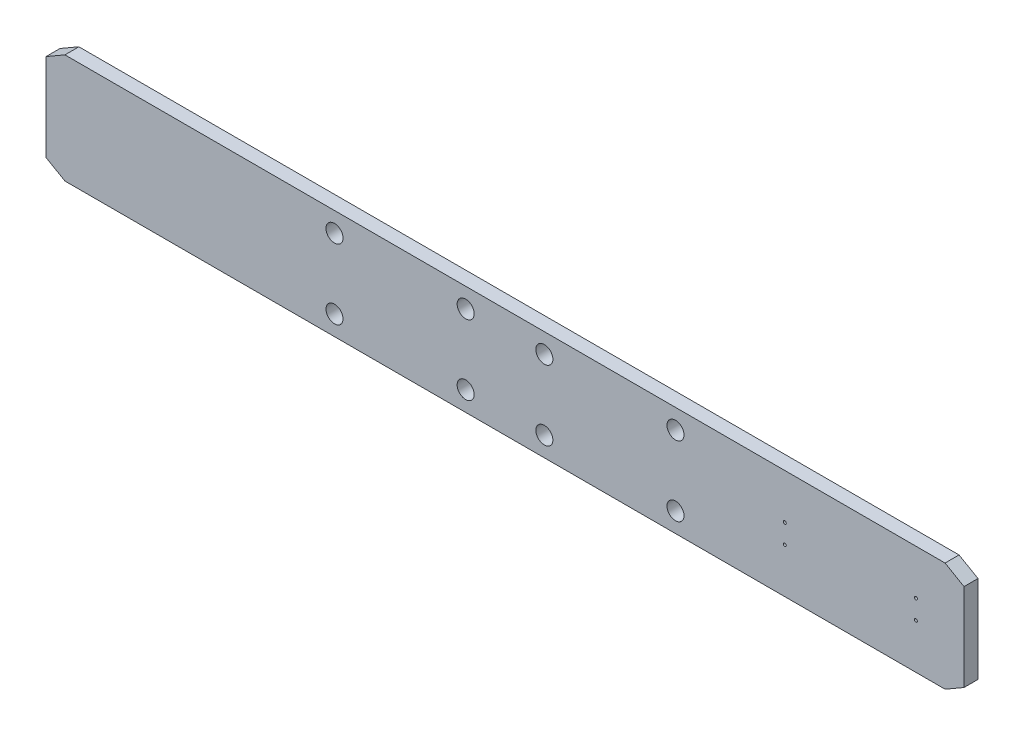
SolidWorks part; units mm, degrees
material "Q235"
ref_plane "Front Plane" through (0, 0, 0) normal (0, 0, 1) x (1, 0, 0)
ref_plane "Top Plane" through (0, 0, 0) normal (0, 1, 0) x (1, 0, 0)
ref_plane "Right Plane" through (0, 0, 0) normal (1, 0, 0) x (0, 0, -1)
sketch "Sketch1" plane through (0, 0, 0) normal (0, 0, 1) x (1, 0, 0)
  line L0 (1050, 100) -> (1006.6987, 125)
  line L1 (-1006.6987, 125) -> (1006.6987, 125)
  line L2 (-1050, 100) -> (-1050, -100)
  line L3 (-1006.6987, -125) -> (1006.6987, -125)
  line L4 (1050, 100) -> (1050, -100)
  line L5 (-1626.1669, 0) -> (1772.2188, 0) construction
  line L6 (1050, -100) -> (1006.6987, -125)
  line L7 (0, 767.823) -> (0, -407.5973) construction
  line L8 (-1050, -100) -> (-1006.6987, -125)
  line L9 (-1050, 100) -> (-1006.6987, 125)
  line L10 (-390, 225.1688) -> (-390, -225.4243) construction
  line L11 (-90, 206.5352) -> (-90, -225.4243) construction
  line L12 (-433.1473, 80) -> (-47.9072, 80) construction
  line L13 (-433.1473, -80) -> (-47.9072, -80) construction
  circle A0 centre (-390, 80) radius 19.5
  circle A1 centre (-90, 80) radius 19.5
  circle A2 centre (-90, -80) radius 19.5
  circle A3 centre (-390, -80) radius 19.5
  circle A4 centre (390, -80) radius 19.5
  circle A5 centre (90, -80) radius 19.5
  circle A6 centre (90, 80) radius 19.5
  circle A7 centre (390, 80) radius 19.5
  dimension "D9" = 39
  dimension "D10" = 39
  dimension "D1" = 300
  dimension "D2" = 125
  dimension "D3" = 2100
  dimension "D4" = 390
  dimension "D5" = 100
  dimension "D6" = 30
  dimension "D7" = 80
  dimension "D8" = 160
extrude "Boss-Extrude1" add sketch "Sketch1" along normal mid plane 32
hole_wizard "M8 Tapped Hole1" positions "Sketch10" profile "Sketch9" tap size "M8" standard "GB" end condition up to next
sketch "Sketch10" plane through (0, 0, 16) normal (0, 0, 1) x (1, 0, 0)
  point P0 (640, 22)
  dimension "D1" = 22
  dimension "D2" = 640
sketch "Sketch9" plane through (640, 22, 16) normal (1, 0, 0) x (0, -1, 0)
  line L0 (0, 0) -> (0, 32)
  line L1 (0, 32) -> (3.4, 32)
  line L2 (3.4, 32) -> (3.4, 0)
  line L5 (3.4, 0) -> (0, 0)
  line L11 (0, -6.35) -> (0, 107.95) construction
  dimension "通孔螺纹孔钻头直径" = 6.8
  dimension "通孔螺纹孔钻头深度" = 32
cosmetic thread "Cosmetic Thread1" parameters "D2"=8
pattern_linear "LPattern1" count 2 spacing 300 along (1, 0, 0) count 2 spacing 44 along (0, -1, 0) of "M8 Tapped Hole1"
